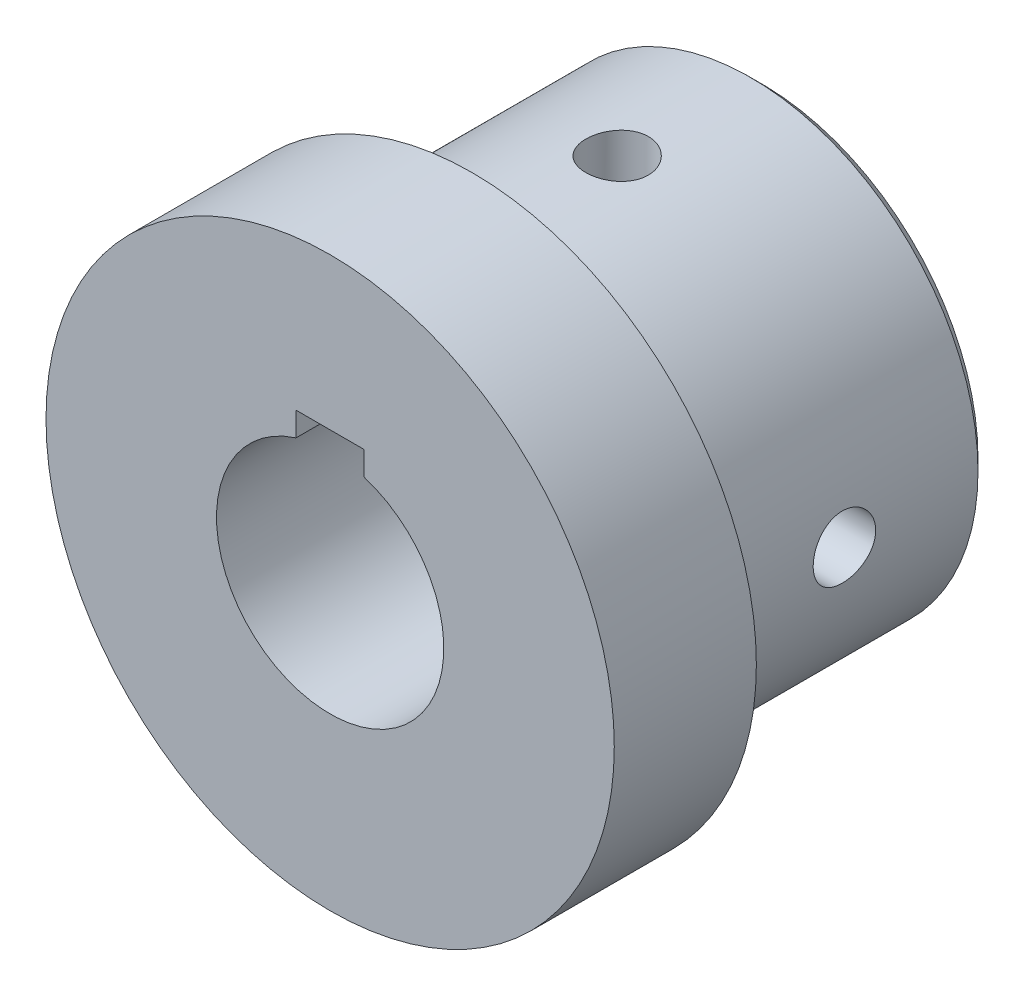
from build123d import *

# Parameters (mm, degrees)
CHAMFER_1_SIZE           = 2
CHAMFER_2_SIZE           = 2
SKETCH_8_R               = 30
SKETCH_8_R_2             = 20
EXTRUDE_1_DEPTH          = 76
SKETCH_9_W               = 12
SKETCH_9_H               = 4.221215972
CUT_EXTRUDE_1_DEPTH      = 104.807514179
SKETCH_11_W              = 2.5
SKETCH_11_H              = 26.7
PATTERN_CIRCULAR_2_COUNT = 4
SKETCH_14_R              = 5.5
CUT_EXTRUDE_2_DEPTH      = 8
PATTERN_CIRCULAR_3_COUNT = 4


with BuildPart() as part:
    # 草图1 → 旋转1 (revolve)
    with BuildSketch(Plane(origin=(0, 0, 0), x_dir=(0, 0, -1), z_dir=(1, 0, 0)), mode=Mode.PRIVATE) as revolve_1_sk:
        Polygon((0, 21), (0, 40), (-51, 40), (-51, 50), (-76, 50), (-76, 30), (-16, 30), (-16, 21), align=None)
    revolve(revolve_1_sk.sketch.rotate(Axis((0, 0, 0), (0, 0, -1)), 90), axis=Axis((0, 0, 0), (0, 0, -1)))

    # 倒角1
    chamfer_1_edges = [part.edges().sort_by_distance(p)[0] for p in [
        (-40, 0, 51),
    ]]
    chamfer(chamfer_1_edges, length=CHAMFER_1_SIZE)

    # 倒角2
    chamfer_2_edges = [part.edges().sort_by_distance(p)[0] for p in [
        (-40, 0, 0),
    ]]
    chamfer(chamfer_2_edges, length=CHAMFER_2_SIZE)

    # 草图8 → 凸台-拉伸1 (add, through all)
    with BuildSketch(Plane.XY.offset(76)):
        Circle(SKETCH_8_R)
        Circle(SKETCH_8_R_2, mode=Mode.SUBTRACT)
    extrude(amount=-EXTRUDE_1_DEPTH)

    # 草图9 → 切除-拉伸1 (cut, through all)
    with BuildSketch(Plane(origin=(0, 0, 0), x_dir=(-1, 0, 0), z_dir=(0, 0, -1))):
        with Locations((0, 21.189392014)):
            Rectangle(SKETCH_9_W, SKETCH_9_H)
    extrude(amount=-CUT_EXTRUDE_1_DEPTH, mode=Mode.SUBTRACT)

    # 草图11 → M6 螺纹孔1 (revolve, cut)
    with BuildSketch(Plane(origin=(0, 23.3, 25.5), x_dir=(0, 0, -1), z_dir=(1, 0, 0))):
        with Locations((1.25, 13.35)):
            Rectangle(SKETCH_11_W, SKETCH_11_H)
    hole_wizard_m6_1 = revolve(axis=Axis((0, 16.95, 25.5), (0, 1, 0)), mode=Mode.SUBTRACT)

    # 阵列(圆周)2: M6 螺纹孔1 ×4 about axis
    pattern_circular_2_axis = Axis((0, 0, 0), (0, 0, 1))
    for i in range(1, PATTERN_CIRCULAR_2_COUNT):
        add(hole_wizard_m6_1.rotate(pattern_circular_2_axis, i * 360 / PATTERN_CIRCULAR_2_COUNT), mode=Mode.SUBTRACT)

    # 草图14 → 切除-拉伸2 (cut)
    with BuildSketch(Plane.ZY.offset(40)):
        with Locations((25.5, 0)):
            Circle(SKETCH_14_R)
    cut_extrude_2 = extrude(amount=-CUT_EXTRUDE_2_DEPTH, mode=Mode.SUBTRACT)

    # 阵列(圆周)3: 切除-拉伸2 ×4 about axis
    pattern_circular_3_axis = Axis((0, 0, 0), (0, 0, 1))
    for i in range(1, PATTERN_CIRCULAR_3_COUNT):
        add(cut_extrude_2.rotate(pattern_circular_3_axis, i * 360 / PATTERN_CIRCULAR_3_COUNT), mode=Mode.SUBTRACT)


solid = part.part
